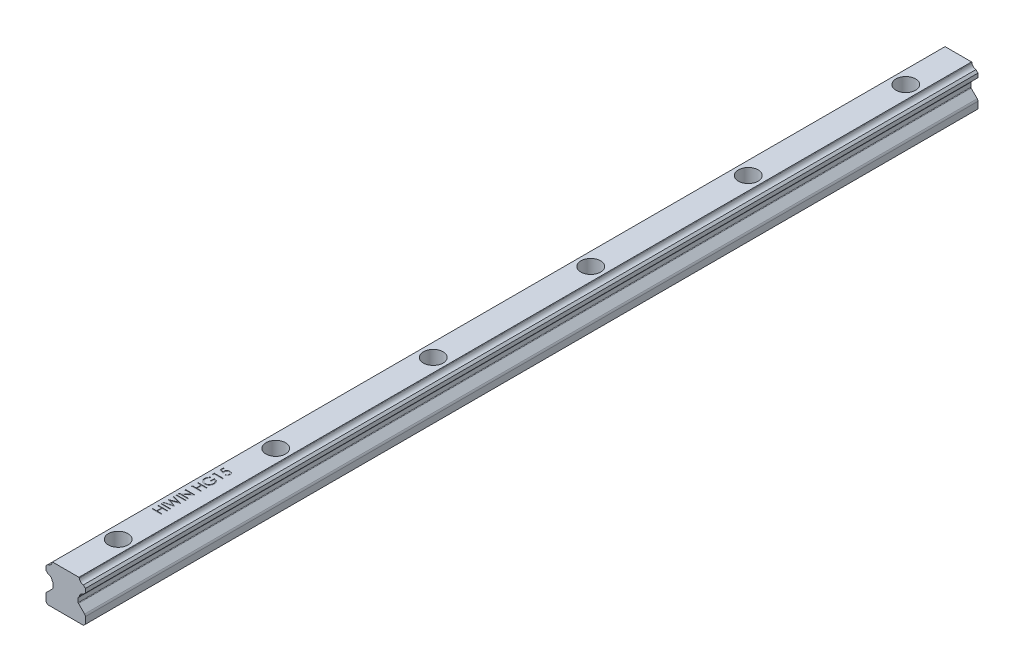
from build123d import *

# Parameters (mm, degrees)
BOSS_EXTRUDE1_DEPTH                                 = 340
CBORE_FOR_M4_HEX_SOCKET_HEAD_CAP_SCREW1_D           = 4.5
CBORE_FOR_M4_HEX_SOCKET_HEAD_CAP_SCREW1_CBORE_D     = 7.5
CBORE_FOR_M4_HEX_SOCKET_HEAD_CAP_SCREW1_CBORE_DEPTH = 5.3
LPATTERN1_COUNT                                     = 6
LPATTERN1_PITCH                                     = 60
SKETCH6_W                                           = 3.5
SKETCH6_H                                           = 0.314102564
CUT_EXTRUDE1_DEPTH                                  = 0.1


with BuildPart() as part:
    # Sketch1 → Boss-Extrude1 (new body)
    with BuildSketch(Plane.XY):
        with BuildLine():
            Line((7.5, 12.548994949), (6.730359225, 13.318635725))
            ThreePointArc((6.730359225, 13.318635725), (5.723905866, 13.746099326), (5.218323295, 14.715666114))
            ThreePointArc((5.218323295, 14.715666114), (5.180299299, 14.839173933), (5.104881891, 14.944113058))
            Line((5.104881891, 14.944113058), (5.04899495, 15))
            Line((5.04899495, 15), (-5.04899495, 15))
            Line((-5.04899495, 15), (-5.104881891, 14.944113058))
            ThreePointArc((-5.104881891, 14.944113058), (-5.180299299, 14.839173933), (-5.218323294, 14.715666114))
            ThreePointArc((-5.218323294, 14.715666114), (-5.723905866, 13.746099326), (-6.730359225, 13.318635725))
            Line((-6.730359225, 13.318635725), (-7.5, 12.548994949))
            Line((-7.5, 12.548994949), (-7.5, 11.011005051))
            Line((-7.5, 11.011005051), (-6.741857404, 10.252862454))
            ThreePointArc((-6.741857404, 10.252862454), (-5.724401564, 9.825237084), (-5.216972518, 8.845137289))
            ThreePointArc((-5.216972518, 8.845137289), (-5.179171399, 8.720266667), (-5.10319759, 8.614202641))
            Line((-5.10319759, 8.614202641), (-4.887157287, 8.398162338))
            ThreePointArc((-4.887157287, 8.398162338), (-4.800448187, 8.268392999), (-4.77, 8.115319626))
            Line((-4.77, 8.115319626), (-4.77, 6.553259018))
            ThreePointArc((-4.77, 6.553259018), (-4.800448187, 6.400185645), (-4.887157287, 6.270416306))
            Line((-4.887157287, 6.270416306), (-7.207106781, 3.950466812))
            ThreePointArc((-7.207106781, 3.950466812), (-7.423879533, 3.626043463), (-7.5, 3.243360031))
            Line((-7.5, 3.243360031), (-7.5, 0.7))
            Line((-7.5, 0.7), (-6.8, 0))
            Line((-6.8, 0), (6.8, 0))
            Line((6.8, 0), (7.5, 0.7))
            Line((7.5, 0.7), (7.5, 3.243360031))
            ThreePointArc((7.5, 3.243360031), (7.423879533, 3.626043463), (7.207106781, 3.950466812))
            Line((7.207106781, 3.950466812), (4.887157287, 6.270416306))
            ThreePointArc((4.887157287, 6.270416306), (4.800448187, 6.400185645), (4.77, 6.553259018))
            Line((4.77, 6.553259018), (4.77, 8.115319626))
            ThreePointArc((4.77, 8.115319626), (4.800448187, 8.268392999), (4.887157287, 8.398162338))
            Line((4.887157287, 8.398162338), (5.10319759, 8.614202641))
            ThreePointArc((5.10319759, 8.614202641), (5.179171399, 8.720266667), (5.216972518, 8.845137289))
            ThreePointArc((5.216972518, 8.845137289), (5.724401564, 9.825237084), (6.741857404, 10.252862454))
            Line((6.741857404, 10.252862454), (7.5, 11.011005051))
            Line((7.5, 11.011005051), (7.5, 12.548994949))
        make_face()
    extrude(amount=-BOSS_EXTRUDE1_DEPTH)

    # CBORE for M4 Hex Socket Head Cap Screw1 (through all)
    with Locations(Plane(origin=(0.291487344, 15, -3.466272926), x_dir=(-1, 0, 0), z_dir=(0, 1, 0))):
        with Locations((0.291487344, -16.533727074)):
            cbore_for_m4_hex_socket_head_cap_screw1 = CounterBoreHole(CBORE_FOR_M4_HEX_SOCKET_HEAD_CAP_SCREW1_D / 2, CBORE_FOR_M4_HEX_SOCKET_HEAD_CAP_SCREW1_CBORE_D / 2, CBORE_FOR_M4_HEX_SOCKET_HEAD_CAP_SCREW1_CBORE_DEPTH)

    # LPattern1: CBORE for M4 Hex Socket Head Cap Screw1 ×6
    with Locations(*[(0, 0, -i * LPATTERN1_PITCH) for i in range(1, LPATTERN1_COUNT)]):
        add(cbore_for_m4_hex_socket_head_cap_screw1, mode=Mode.SUBTRACT)

    # Sketch6 → Cut-Extrude1 (cut)
    with BuildSketch(Plane(origin=(0, 15, 0), x_dir=(1, 0, 0), z_dir=(0, 1, 0))):
        Polygon((-3.5, 36.403846154), (-3.5, 36.717948718), (-2.064102564, 36.717948718), (-2.064102564, 38.512820513), (-3.5, 38.512820513), (-3.5, 38.826923077), (0, 38.826923077), (0, 38.512820513), (-1.705128205, 38.512820513), (-1.705128205, 36.717948718), (0, 36.717948718), (0, 36.403846154), align=None)
        with Locations((-1.75, 39.881410256)):
            Rectangle(SKETCH6_W, SKETCH6_H)
        Polygon((-3.5, 40.576923077), (-3.5, 40.901542468), (-0.933193109, 41.586538462), (-3.5, 42.605268429), (-3.5, 42.650841346), (-0.950721154, 43.650641026), (-3.5, 44.339142628), (-3.5, 44.66025641), (0, 43.716546474), (0, 43.671674679), (-2.676883013, 42.618589744), (0, 41.552884615), (0, 41.508012821), align=None)
        with Locations((-1.75, 45.625)):
            Rectangle(SKETCH6_W, SKETCH6_H)
        Polygon((0, 46.544871795), (-3.5, 46.544871795), (-3.5, 46.610777244), (-0.745292468, 48.923076923), (-3.5, 48.923076923), (-3.5, 49.237179487), (0, 49.237179487), (0, 49.165665064), (-2.748397436, 46.858974359), (0, 46.858974359), align=None)
        Polygon((-3.5, 51.480769231), (-3.5, 51.794871795), (-2.064102564, 51.794871795), (-2.064102564, 53.58974359), (-3.5, 53.58974359), (-3.5, 53.903846154), (0, 53.903846154), (0, 53.58974359), (-1.705128205, 53.58974359), (-1.705128205, 51.794871795), (0, 51.794871795), (0, 51.480769231), align=None)
        with BuildLine():
            Line((-2.902644231, 58.076923077), (-2.647435897, 57.807692308))
            add(Edge.make_bspline(
                [(-2.647435897, 57.807692308), (-2.69328212, 57.758983227), (-2.783881335, 57.662726562), (-2.901244074, 57.50552662), (-3.002777003, 57.342170767), (-3.084772592, 57.172394867), (-3.149094254, 57.000650867), (-3.195850217, 56.829891913), (-3.225460377, 56.661223615), (-3.229016796, 56.549059313), (-3.230769231, 56.493790064)],
                knots=[0, 0, 0, 0, 1.089067066, 2.152164705, 3.18986567, 4.218445106, 5.218487318, 6.173592265, 7.100032889, 8, 8, 8, 8], degree=3))
            add(Edge.make_bspline(
                [(-3.230769231, 56.493790064), (-3.230355625, 56.459875364), (-3.229529486, 56.392133924), (-3.218985271, 56.29151198), (-3.203820407, 56.191945342), (-3.181878529, 56.093621968), (-3.15406947, 55.99635068), (-3.119284004, 55.900469793), (-3.078728771, 55.805800421), (-3.031866252, 55.713234402), (-2.980386575, 55.623493669), (-2.923337414, 55.538737672), (-2.862550889, 55.458421211), (-2.796491613, 55.384072004), (-2.725807311, 55.31519549), (-2.651770944, 55.250524789), (-2.572926872, 55.191265211), (-2.489599321, 55.138479571), (-2.403726867, 55.090811977), (-2.316037795, 55.049619777), (-2.227346143, 55.013809823), (-2.136984078, 54.986535862), (-2.045883197, 54.963434988), (-1.953566086, 54.947353752), (-1.859791669, 54.938257435), (-1.796993971, 54.936686944), (-1.765424679, 54.935897436)],
                knots=[0, 0, 0, 0, 1.028150113, 2.053633673, 3.06513288, 4.081487945, 5.106702018, 6.131327874, 7.172780699, 8.228344599, 9.276313556, 10.308389736, 11.324843658, 12.329040066, 13.321460474, 14.316307835, 15.308626991, 16.309440696, 17.305625405, 18.28535951, 19.246194545, 20.203493668, 21.145557131, 22.095268976, 23.042464743, 24, 24, 24, 24], degree=3))
            add(Edge.make_bspline(
                [(-1.765424679, 54.935897436), (-1.733154018, 54.936653631), (-1.668700816, 54.938163957), (-1.572504414, 54.947817154), (-1.477747832, 54.965772364), (-1.384282029, 54.989584114), (-1.291920993, 55.019856789), (-1.20076111, 55.057049303), (-1.110811241, 55.101355435), (-1.022964324, 55.152526704), (-0.937464192, 55.209036172), (-0.856251713, 55.271187356), (-0.780271995, 55.339084893), (-0.708415252, 55.411483836), (-0.641134974, 55.489043832), (-0.579242122, 55.572517364), (-0.521779643, 55.660735956), (-0.469378807, 55.753738745), (-0.42257144, 55.850542725), (-0.38094723, 55.949799156), (-0.346667976, 56.051827058), (-0.31872985, 56.156089724), (-0.295829559, 56.262463002), (-0.281097077, 56.371486803), (-0.270406246, 56.482359512), (-0.269624576, 56.557098144), (-0.269230769, 56.594751603)],
                knots=[0, 0, 0, 0, 0.935915162, 1.869274651, 2.799799983, 3.730201895, 4.664668062, 5.616159355, 6.583070886, 7.570012957, 8.562524459, 9.553461134, 10.53281078, 11.515274572, 12.509912756, 13.507571325, 14.526460018, 15.561318395, 16.601025881, 17.643204557, 18.680545676, 19.719612342, 20.772381578, 21.833430283, 22.908478249, 24, 24, 24, 24], degree=3))
            add(Edge.make_bspline(
                [(-0.269230769, 56.594751603), (-0.270178952, 56.640130135), (-0.272040863, 56.729238255), (-0.286546735, 56.860222075), (-0.309173205, 56.986034693), (-0.342412256, 57.106266531), (-0.384484705, 57.221353926), (-0.436513285, 57.330872414), (-0.497950569, 57.435124408), (-0.567552463, 57.533658668), (-0.645100929, 57.624132689), (-0.728035637, 57.706474768), (-0.817431068, 57.77785339), (-0.911954918, 57.840400707), (-1.012511326, 57.892097951), (-1.118540888, 57.934543829), (-1.230109213, 57.967076285), (-1.307200733, 57.980431374), (-1.346153846, 57.987179487)],
                knots=[0, 0, 0, 0, 1.130199668, 2.219330667, 3.279027493, 4.311506524, 5.322739849, 6.327972234, 7.327472899, 8.33386792, 9.329086447, 10.29244429, 11.240784345, 12.174119183, 13.111530729, 14.052100829, 15.015757696, 16, 16, 16, 16], degree=3))
            Line((-1.346153846, 57.987179487), (-1.346153846, 56.820512821))
            Line((-1.346153846, 56.820512821), (-1.705128205, 56.820512821))
            Line((-1.705128205, 56.820512821), (-1.705128205, 58.301282051))
            add(Edge.make_bspline(
                [(-1.705128205, 58.301282051), (-1.638220716, 58.299576203), (-1.507270675, 58.296237549), (-1.316300404, 58.272818634), (-1.13592871, 58.235002122), (-0.965965639, 58.18334181), (-0.806652046, 58.116466529), (-0.65782618, 58.035094001), (-0.520449499, 57.93792188), (-0.393400495, 57.828411438), (-0.280071283, 57.705511481), (-0.180465345, 57.572542861), (-0.09656273, 57.429285892), (-0.028302067, 57.275876085), (0.024971927, 57.112815651), (0.062743504, 56.939727272), (0.085373467, 56.756845671), (0.088264847, 56.631508994), (0.08974359, 56.567407853)],
                knots=[0, 0, 0, 0, 1.140356446, 2.231883559, 3.274166699, 4.278491846, 5.25512956, 6.21435461, 7.1637429, 8.11826594, 9.068280886, 10.0076534, 10.945064095, 11.891975133, 12.864533718, 13.863980011, 14.907571808, 16, 16, 16, 16], degree=3))
            add(Edge.make_bspline(
                [(0.08974359, 56.567407853), (0.089174469, 56.527897717), (0.088051978, 56.449970996), (0.080074631, 56.334880068), (0.067794054, 56.222962448), (0.049248931, 56.114234439), (0.026534277, 56.008296097), (-0.002552442, 55.905676512), (-0.036221141, 55.80598477), (-0.074516815, 55.709066784), (-0.118888472, 55.615802237), (-0.168198111, 55.52577572), (-0.222191472, 55.438489595), (-0.281802318, 55.35453843), (-0.346584778, 55.273484808), (-0.416668697, 55.195851364), (-0.491839816, 55.121203486), (-0.545218826, 55.074443023), (-0.572115385, 55.05088141)],
                knots=[0, 0, 0, 0, 1.107784379, 2.184907829, 3.233506516, 4.263428166, 5.276301166, 6.270063455, 7.25232949, 8.225834625, 9.190232166, 10.146266622, 11.1027726, 12.066435141, 13.031522626, 14.010570082, 14.99756817, 16, 16, 16, 16], degree=3))
            add(Edge.make_bspline(
                [(-0.572115385, 55.05088141), (-0.614786038, 55.016695478), (-0.699419055, 54.948891066), (-0.835018999, 54.861612909), (-0.975420859, 54.787211506), (-1.121015488, 54.726843684), (-1.271666701, 54.679705598), (-1.427181992, 54.645899345), (-1.587761622, 54.626092056), (-1.696426887, 54.623238518), (-1.751402244, 54.621794872)],
                knots=[0, 0, 0, 0, 1.023165419, 2.029347347, 3.013907458, 3.994755782, 4.975994455, 5.96558838, 6.970761222, 8, 8, 8, 8], degree=3))
            add(Edge.make_bspline(
                [(-1.751402244, 54.621794872), (-1.792568496, 54.62232711), (-1.874377804, 54.623384821), (-1.99583511, 54.636210339), (-2.115135808, 54.654611751), (-2.232182344, 54.681658827), (-2.347053012, 54.715755013), (-2.45980069, 54.758308794), (-2.570493643, 54.807852572), (-2.67836343, 54.865442289), (-2.782003044, 54.929511026), (-2.880905313, 54.999118682), (-2.973467332, 55.074802367), (-3.059903521, 55.156782462), (-3.141494975, 55.243406392), (-3.216537375, 55.336492693), (-3.286205011, 55.434631029), (-3.349159221, 55.538582169), (-3.405727075, 55.6467058), (-3.455315154, 55.758766886), (-3.496298775, 55.874724704), (-3.531072472, 55.993712261), (-3.556787635, 56.11662974), (-3.575436374, 56.242585283), (-3.588196976, 56.372235393), (-3.589223231, 56.459871423), (-3.58974359, 56.504306891)],
                knots=[0, 0, 0, 0, 1.00895651, 2.005089799, 2.991467152, 3.967318338, 4.948153826, 5.927364234, 6.919980553, 7.91976625, 8.923240147, 9.905815003, 10.88314567, 11.851989312, 12.825009789, 13.798721852, 14.781296708, 15.773896486, 16.776076962, 17.771600213, 18.775744723, 19.78957137, 20.808953803, 21.851964491, 22.910847925, 24, 24, 24, 24], degree=3))
            add(Edge.make_bspline(
                [(-3.58974359, 56.504306891), (-3.589164098, 56.540545135), (-3.588015034, 56.612401313), (-3.580050386, 56.719327046), (-3.567426505, 56.82460006), (-3.550199718, 56.92837645), (-3.526736028, 57.030302816), (-3.498657743, 57.130669522), (-3.46596592, 57.229622058), (-3.426977074, 57.326850307), (-3.382723449, 57.423008023), (-3.332910027, 57.518629864), (-3.276685022, 57.61338911), (-3.213881487, 57.707450091), (-3.145578069, 57.801405949), (-3.069821245, 57.893770591), (-2.989598489, 57.986773536), (-2.931916305, 58.04657535), (-2.902644231, 58.076923077)],
                knots=[0, 0, 0, 0, 0.985871117, 1.954866573, 2.915460327, 3.869826059, 4.81536089, 5.759505086, 6.70452669, 7.649098992, 8.607881297, 9.583363685, 10.581137262, 11.603961102, 12.659522466, 13.73993555, 14.853081303, 16, 16, 16, 16], degree=3))
        make_face()
        Polygon((-3.5, 59.449018429), (-3.5, 60.096153846), (0, 60.096153846), (0, 59.782051282), (-3.141025641, 59.782051282), (-3.141025641, 59.243589744), align=None)
        with BuildLine():
            Line((-3.5, 63.596153846), (-3.141025641, 63.596153846))
            Line((-3.141025641, 63.596153846), (-3.141025641, 62.405649038))
            Line((-3.141025641, 62.405649038), (-2.220452724, 62.217047276))
            add(Edge.make_bspline(
                [(-2.220452724, 62.217047276), (-2.230682996, 62.25410315), (-2.25050253, 62.325893046), (-2.2725083, 62.431852907), (-2.285773744, 62.53244511), (-2.287585055, 62.597720481), (-2.288461538, 62.629306891)],
                knots=[0, 0, 0, 0, 1.100273476, 2.13160584, 3.095893838, 4, 4, 4, 4], degree=3))
            add(Edge.make_bspline(
                [(-2.288461538, 62.629306891), (-2.28764354, 62.668397805), (-2.28603515, 62.745260309), (-2.269673986, 62.857544614), (-2.245976174, 62.96527195), (-2.209465207, 63.066851732), (-2.164878805, 63.163891055), (-2.108721258, 63.254723386), (-2.04315746, 63.34062356), (-1.968525078, 63.420997879), (-1.885534459, 63.493570878), (-1.795933934, 63.556634421), (-1.701678739, 63.611677196), (-1.600559725, 63.654605621), (-1.494484031, 63.689639403), (-1.382227183, 63.712740767), (-1.264785773, 63.728171477), (-1.18448027, 63.729891917), (-1.143529647, 63.730769231)],
                knots=[0, 0, 0, 0, 1.052805225, 2.070078116, 3.052532748, 4.020689046, 4.973125432, 5.925915817, 6.89216474, 7.881560752, 8.877013184, 9.857446635, 10.830895175, 11.812622661, 12.812548702, 13.836681939, 14.896847428, 16, 16, 16, 16], degree=3))
            add(Edge.make_bspline(
                [(-1.143529647, 63.730769231), (-1.115007605, 63.730103556), (-1.058348972, 63.728781204), (-0.974202158, 63.7220714), (-0.891849045, 63.709103007), (-0.811440613, 63.69190289), (-0.732901554, 63.668941583), (-0.65579213, 63.642084161), (-0.580956685, 63.608702163), (-0.508064701, 63.571694489), (-0.437950402, 63.530715464), (-0.372294905, 63.484635462), (-0.309599937, 63.436755685), (-0.251727444, 63.384438189), (-0.198452948, 63.328277796), (-0.149513072, 63.268586987), (-0.104029493, 63.205907167), (-0.063861909, 63.139251137), (-0.026898788, 63.070108867), (0.003424705, 62.997480593), (0.030535245, 62.923019908), (0.05214477, 62.845655028), (0.069077325, 62.765561217), (0.080577925, 62.682606441), (0.088954363, 62.597225771), (0.08947872, 62.539350758), (0.08974359, 62.510116186)],
                knots=[0, 0, 0, 0, 1.056393913, 2.098511576, 3.122979385, 4.141471433, 5.141222888, 6.151259816, 7.162667642, 8.172852865, 9.177685681, 10.166741883, 11.141342384, 12.097242845, 13.052202613, 14.005160326, 14.953864445, 15.917140761, 16.884916217, 17.854238259, 18.828761908, 19.81781811, 20.826036654, 21.857789401, 22.917898972, 24, 24, 24, 24], degree=3))
            add(Edge.make_bspline(
                [(0.08974359, 62.510116186), (0.089050894, 62.475242894), (0.087688097, 62.406633813), (0.073496095, 62.30610057), (0.053035464, 62.209432256), (0.022721931, 62.117043177), (-0.016971483, 62.029318648), (-0.064133263, 61.945002475), (-0.12027864, 61.865139718), (-0.184894072, 61.790276377), (-0.255892818, 61.721460371), (-0.332202561, 61.65905751), (-0.413920487, 61.604193873), (-0.500780871, 61.556670445), (-0.592629648, 61.516184815), (-0.689749822, 61.484366409), (-0.791650601, 61.45868899), (-0.861804004, 61.447825441), (-0.897435897, 61.442307692)],
                knots=[0, 0, 0, 0, 1.046872515, 2.059598001, 3.044168548, 4.012104806, 4.973680974, 5.932408326, 6.910122221, 7.900780896, 8.89867654, 9.876692837, 10.858029398, 11.85084981, 12.847361615, 13.868568023, 14.917415949, 16, 16, 16, 16], degree=3))
            Line((-0.897435897, 61.442307692), (-0.897435897, 61.756410256))
            add(Edge.make_bspline(
                [(-0.897435897, 61.756410256), (-0.86405597, 61.764133979), (-0.799897896, 61.778979402), (-0.709812799, 61.811649494), (-0.62950762, 61.851206459), (-0.558491359, 61.899340396), (-0.495464081, 61.955133792), (-0.43989307, 62.019990731), (-0.389697273, 62.092289811), (-0.347784769, 62.17267219), (-0.312479137, 62.257640252), (-0.287283878, 62.346063351), (-0.272032646, 62.436668904), (-0.270168243, 62.497671524), (-0.269230769, 62.528345353)],
                knots=[0, 0, 0, 0, 1.13623081, 2.183898708, 3.172478118, 4.09966615, 5.022692284, 5.957376522, 6.927682873, 7.937366477, 8.960015386, 9.976409503, 10.982481913, 12, 12, 12, 12], degree=3))
            add(Edge.make_bspline(
                [(-0.269230769, 62.528345353), (-0.270058415, 62.558301256), (-0.271688055, 62.617284674), (-0.284028564, 62.704132513), (-0.303533592, 62.787735767), (-0.33085902, 62.868242843), (-0.367008958, 62.945258145), (-0.411417074, 63.018672781), (-0.462975425, 63.089532607), (-0.521904738, 63.1559727), (-0.586881759, 63.216808942), (-0.656357238, 63.270565902), (-0.730474586, 63.315342595), (-0.807947606, 63.353076763), (-0.889626199, 63.381730046), (-0.975127364, 63.402171031), (-1.064662347, 63.414174089), (-1.125731657, 63.415825269), (-1.156850962, 63.416666667)],
                knots=[0, 0, 0, 0, 1.027268864, 2.022700798, 3.002744649, 3.968653148, 4.933396556, 5.915045722, 6.907600446, 7.935526002, 8.956456544, 9.95700807, 10.942805781, 11.92166854, 12.907987664, 13.905483474, 14.932689774, 16, 16, 16, 16], degree=3))
            add(Edge.make_bspline(
                [(-1.156850962, 63.416666667), (-1.184930032, 63.416028195), (-1.239659043, 63.414783746), (-1.320009695, 63.404010642), (-1.396158478, 63.386014341), (-1.468436727, 63.360391264), (-1.536613353, 63.328412845), (-1.600538112, 63.288262971), (-1.660812066, 63.241651258), (-1.715884112, 63.187233139), (-1.766793088, 63.12803749), (-1.810034281, 63.062543866), (-1.846807397, 62.992500701), (-1.876936465, 62.917778197), (-1.900936575, 62.838284311), (-1.917523378, 62.753976228), (-1.92744867, 62.664834733), (-1.928795087, 62.603859089), (-1.929487179, 62.572516026)],
                knots=[0, 0, 0, 0, 1.045723156, 2.038222538, 3.013889863, 3.95567481, 4.890389958, 5.81331128, 6.76251276, 7.723027653, 8.692928204, 9.666105983, 10.639751036, 11.635719707, 12.66315958, 13.728667616, 14.832476222, 16, 16, 16, 16], degree=3))
            add(Edge.make_bspline(
                [(-1.929487179, 62.572516026), (-1.928906588, 62.545387097), (-1.927707815, 62.489372742), (-1.918881318, 62.403449915), (-1.904642024, 62.313158192), (-1.885055776, 62.218843696), (-1.859424699, 62.120223188), (-1.828710199, 62.017504787), (-1.7919882, 61.910472521), (-1.764255986, 61.838354796), (-1.75, 61.801282051)],
                knots=[0, 0, 0, 0, 0.817624296, 1.688186739, 2.600797293, 3.572016777, 4.590301741, 5.671205678, 6.80286297, 8, 8, 8, 8], degree=3))
            Line((-1.75, 61.801282051), (-3.5, 62.16025641))
            Line((-3.5, 62.16025641), (-3.5, 63.596153846))
        make_face()
    extrude(amount=-CUT_EXTRUDE1_DEPTH, mode=Mode.SUBTRACT)


solid = part.part
